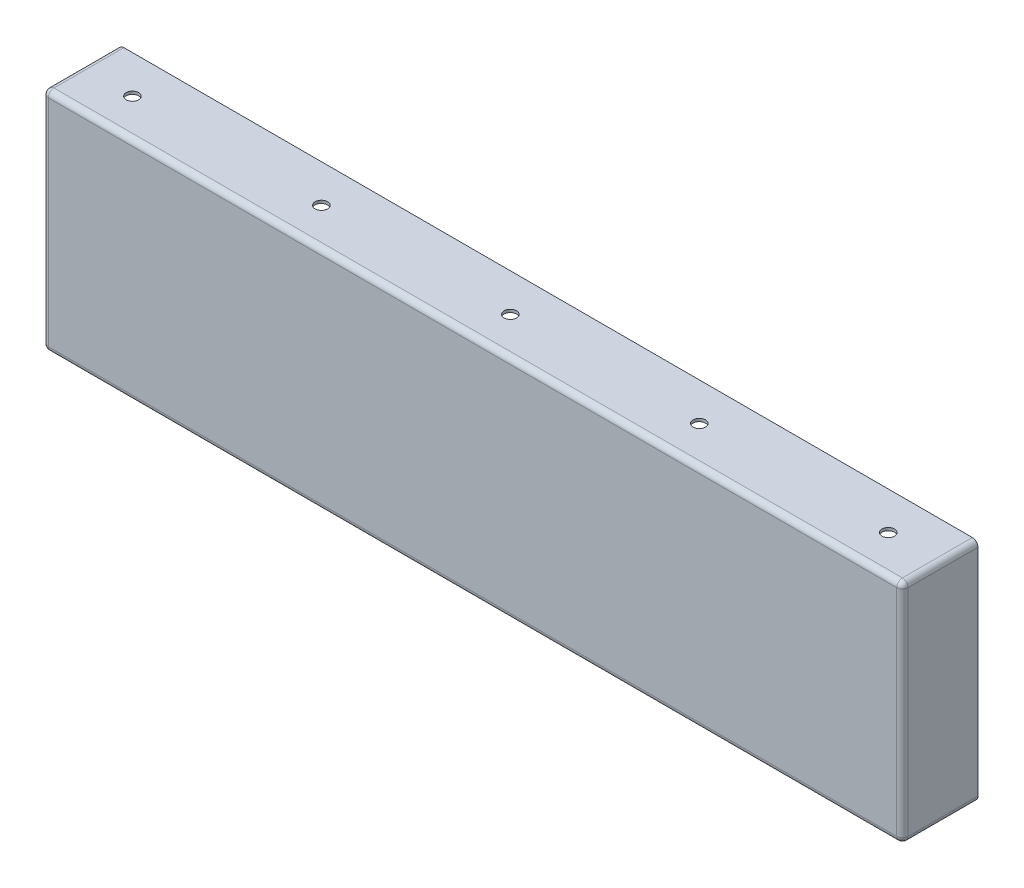
from build123d import *

# Parameters (mm, degrees)
SKETCH_1_W         = 455
SKETCH_1_H         = 120
EXTRUDE_1_DEPTH    = 40
FILLET_1_R         = 3
SHELL_1_T          = -1.5
HOLE_WIZARD_M6_1_D = 6.6


with BuildPart() as part:
    # 草图1 → 凸台-拉伸1 (new body)
    with BuildSketch(Plane.XY):
        Rectangle(SKETCH_1_W, SKETCH_1_H)
    extrude(amount=EXTRUDE_1_DEPTH)

    # 圆角1
    fillet_1_edges = [part.edges().sort_by_distance(p)[0] for p in [
        (-227.5, 0, 40),
        (0, -60, 40),
        (227.5, 0, 40),
        (0, 60, 40),
        (227.5, -60, 20),
        (-227.5, -60, 20),
        (-227.5, 60, 20),
        (227.5, 60, 20),
    ]]
    fillet(fillet_1_edges, radius=FILLET_1_R)

    # 抽壳1
    shell_1_openings = [part.faces().sort_by_distance(p)[0] for p in [
        (0, 0, 0),
    ]]
    offset(amount=SHELL_1_T, openings=shell_1_openings, kind=Kind.INTERSECTION)

    # M6 间隙孔1 (through all)
    with Locations(Plane(origin=(0, -60, 0), x_dir=(-1, 0, 0), z_dir=(0, -1, 0))):
        with Locations((200, -20), (100, -20), (-100, -20), (-200, -20), (0, -20)):
            Hole(HOLE_WIZARD_M6_1_D / 2)


solid = part.part
